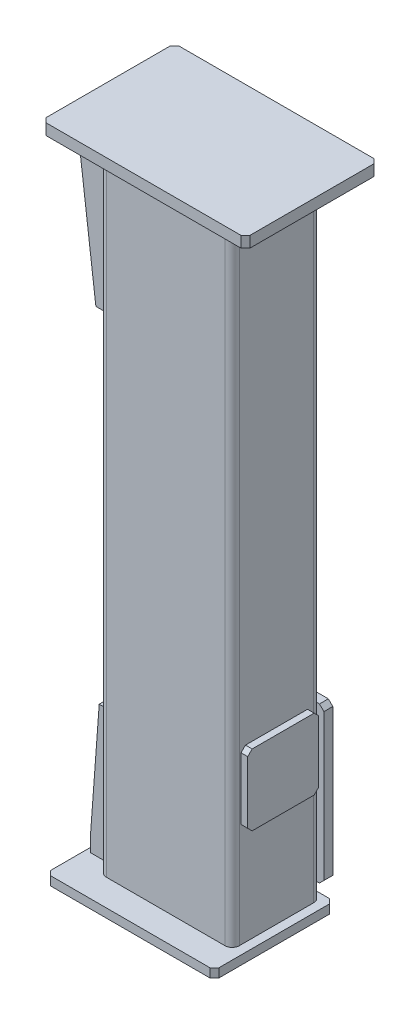
from build123d import *

# Parameters (mm, degrees)
BOSS_EXTRUDE1_DEPTH  = 20
BOSS_EXTRUDE2_DEPTH  = 1431
BOSS_EXTRUDE3_DEPTH  = 25
BOSS_EXTRUDE4_START  = -22.5
BOSS_EXTRUDE4_DEPTH  = 15
BOSS_EXTRUDE5_DEPTH  = 15
BOSS_EXTRUDE9_START  = -30
BOSS_EXTRUDE9_DEPTH  = 15
BOSS_EXTRUDE10_DEPTH = 20


with BuildPart() as part:
    # Sketch1 → Boss-Extrude1 (new body)
    with BuildSketch(Plane(origin=(0, 0, 0), x_dir=(1, 0, 0), z_dir=(0, 1, 0))):
        with BuildLine():
            Line((-3.496816057, 9.368686005), (-3.496816057, 309.368686005))
            Line((-3.496816057, 309.368686005), (6.503183943, 319.368686005))
            Line((6.503183943, 319.368686005), (141.657748152, 319.368686005))
            Line((141.657748152, 319.368686005), (266.503183943, 319.368686005))
            Line((266.503183943, 319.368686005), (276.503183943, 309.368686005))
            Line((276.503183943, 309.368686005), (276.503183943, 274.368686005))
            ThreePointArc((276.503183943, 274.368686005), (277.967650037, 270.833152099), (281.503183943, 269.368686005))
            Line((281.503183943, 269.368686005), (366.503183943, 269.368686005))
            Line((366.503183943, 269.368686005), (376.503183943, 259.368686005))
            Line((376.503183943, 259.368686005), (376.503183943, 9.368686005))
            Line((376.503183943, 9.368686005), (366.503183943, -0.631313995))
            Line((366.503183943, -0.631313995), (6.503183943, -0.631313995))
            Line((6.503183943, -0.631313995), (-3.496816057, 9.368686005))
        make_face()
    extrude(amount=BOSS_EXTRUDE1_DEPTH)

    # Sketch2 → Boss-Extrude2 (add)
    with BuildSketch(Plane(origin=(0, 20, 0), x_dir=(1, 0, 0), z_dir=(0, 1, 0))):
        with BuildLine():
            Line((72.503183943, 259.368686005), (340.503183943, 259.368686005))
            ThreePointArc((340.503183943, 259.368686005), (351.816892442, 254.682394504), (356.503183943, 243.368686005))
            Line((356.503183943, 243.368686005), (356.503183943, 75.368686005))
            ThreePointArc((356.503183943, 75.368686005), (351.816892442, 64.054977506), (340.503183943, 59.368686005))
            Line((340.503183943, 59.368686005), (72.503183943, 59.368686005))
            ThreePointArc((72.503183943, 59.368686005), (61.189475444, 64.054977506), (56.503183943, 75.368686005))
            Line((56.503183943, 75.368686005), (56.503183943, 243.368686005))
            ThreePointArc((56.503183943, 243.368686005), (61.189475444, 254.682394504), (72.503183943, 259.368686005))
        make_face()
        with BuildLine():
            Line((72.503183943, 251.368686005), (340.503183943, 251.368686005))
            ThreePointArc((340.503183943, 251.368686005), (346.160038192, 249.025540255), (348.503183943, 243.368686005))
            Line((348.503183943, 243.368686005), (348.503183943, 75.368686005))
            ThreePointArc((348.503183943, 75.368686005), (346.160038192, 69.711831756), (340.503183943, 67.368686005))
            Line((340.503183943, 67.368686005), (72.503183943, 67.368686005))
            ThreePointArc((72.503183943, 67.368686005), (66.846329693, 69.711831756), (64.503183943, 75.368686005))
            Line((64.503183943, 75.368686005), (64.503183943, 243.368686005))
            ThreePointArc((64.503183943, 243.368686005), (66.846329693, 249.025540255), (72.503183943, 251.368686005))
        make_face(mode=Mode.SUBTRACT)
    extrude(amount=BOSS_EXTRUDE2_DEPTH)

    # Sketch3 → Boss-Extrude3 (add)
    with BuildSketch(Plane(origin=(0, 1451, 0), x_dir=(1, 0, 0), z_dir=(0, 1, 0))):
        Polygon((-13.496816057, 309.368686005), (426.503183943, 309.368686005), (436.503183943, 299.368686005), (436.503183943, 19.368686005), (426.503183943, 9.368686005), (-13.496816057, 9.368686005), (-23.496816057, 19.368686005), (-23.496816057, 299.368686005), align=None)
    extrude(amount=BOSS_EXTRUDE3_DEPTH)

    # Sketch4 → Boss-Extrude4 (add)
    with BuildSketch(Plane.XY.offset(-59.368686005).offset(BOSS_EXTRUDE4_START)):
        Polygon((-13.496816057, 1451), (46.503183943, 1451), (56.503183943, 1441), (56.503183943, 1101), (26.503183943, 1101), (-13.496816057, 1421), align=None)
    boss_extrude4 = extrude(amount=-BOSS_EXTRUDE4_DEPTH)

    # Mirror1: Boss-Extrude4 across plane
    add(boss_extrude4.mirror(Plane.XY.offset(-159.368686005)))

    # Sketch5 → Boss-Extrude5 (add)
    with BuildSketch(Plane(origin=(356.503183943, 0, 0), x_dir=(0, 0, -1), z_dir=(1, 0, 0))):
        Polygon((89.368686005, 405), (229.368686005, 405), (239.368686005, 395), (239.368686005, 255), (229.368686005, 245), (89.368686005, 245), (79.368686005, 255), (79.368686005, 395), align=None)
    extrude(amount=BOSS_EXTRUDE5_DEPTH)

    # Sketch9 → Boss-Extrude9 (add)
    with BuildSketch(Plane.XY.offset(-59.368686005).offset(BOSS_EXTRUDE9_START)):
        Polygon((56.503183943, 30), (56.503183943, 320), (26.503183943, 320), (6.503183943, 50), (6.503183943, 20), (46.503183943, 20), align=None)
    boss_extrude9 = extrude(amount=-BOSS_EXTRUDE9_DEPTH)

    # Mirror2: Boss-Extrude9 across plane
    add(boss_extrude9.mirror(Plane.XY.offset(-159.368686005)))

    # Sketch10 → Boss-Extrude10 (add)
    with BuildSketch(Plane(origin=(0, 0, -259.368686005), x_dir=(-1, 0, 0), z_dir=(0, 0, -1))):
        Polygon((-353.503183943, 399), (-288.503183943, 399), (-278.503183943, 389), (-278.503183943, 59), (-288.503183943, 49), (-353.503183943, 49), (-363.503183943, 59), (-363.503183943, 389), align=None)
    extrude(amount=BOSS_EXTRUDE10_DEPTH)


solid = part.part
